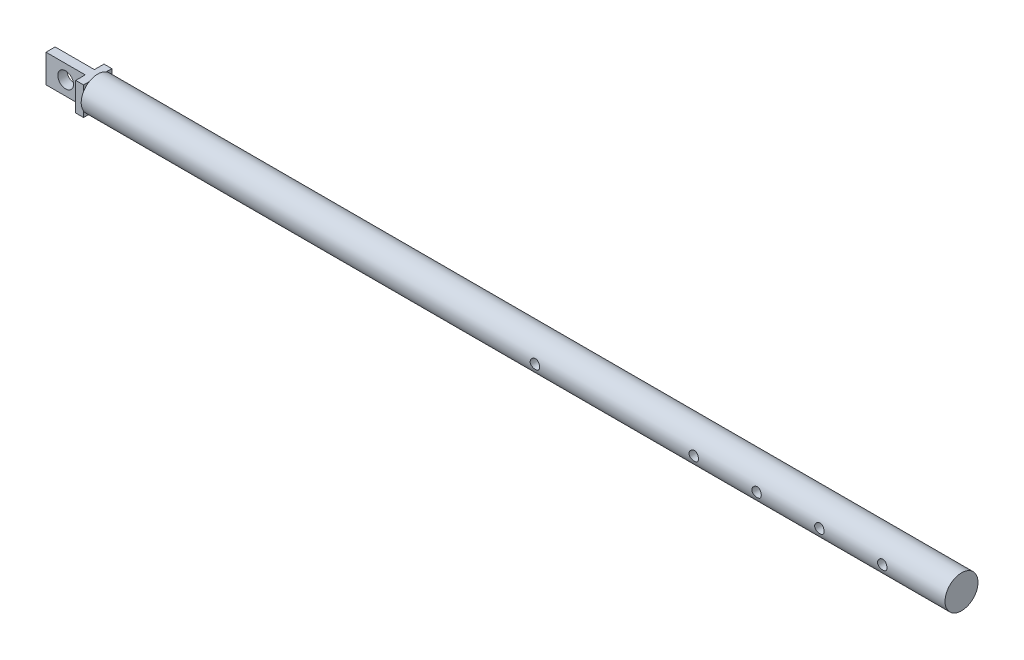
from build123d import *

# Parameters (mm, degrees)
SKETCH_1_W               = 550
SKETCH_1_H               = 10.5
CUT_EXTRUDE_1_DEPTH      = 15
CUT_EXTRUDE_1_DEPTH_BACK = 15
SKETCH_2_R               = 3
SKETCH_10_W              = 18
SKETCH_10_H              = 18
EXTRUDE_3_DEPTH          = 5
SKETCH_11_W              = 5.828442308
SKETCH_11_H              = 18
EXTRUDE_4_DEPTH          = 25
SKETCH_12_R              = 5
CUT_EXTRUDE_2_DEPTH      = 25


with BuildPart() as part:
    # 草图1 → 旋转1 (revolve)
    with BuildSketch(Plane.XY):
        with Locations((-275, 5.25)):
            Rectangle(SKETCH_1_W, SKETCH_1_H)
    revolve(axis=Axis((94.334642974, 0, 0), (-1, 0, 0)))

    # 草图2 → 切除-拉伸1 (cut, two sides: drawn at the far end of the back side and taken through both)
    with BuildSketch(Plane.XY.offset(-CUT_EXTRUDE_1_DEPTH_BACK)):
        with Locations(Location((-40, 0, 0), (0, 0, 180))):
            Circle(SKETCH_2_R)
        with Locations(Location((-80, 0, 0), (0, 0, 180))):
            Circle(SKETCH_2_R)
        with Locations(Location((-120, 0, 0), (0, 0, 180))):
            Circle(SKETCH_2_R)
        with Locations(Location((-160, 0, 0), (0, 0, 180))):
            Circle(SKETCH_2_R)
        with Locations(Location((-261.159789745, 0, 0), (0, 0, 180))):
            Circle(SKETCH_2_R)
    extrude(amount=CUT_EXTRUDE_1_DEPTH + CUT_EXTRUDE_1_DEPTH_BACK, mode=Mode.SUBTRACT)

    # 草图10 → 凸台-拉伸3 (add)
    with BuildSketch(Plane.ZY.offset(550)):
        Rectangle(SKETCH_10_W, SKETCH_10_H)
    extrude(amount=EXTRUDE_3_DEPTH)

    # 草图11 → 凸台-拉伸4 (add)
    with BuildSketch(Plane.ZY.offset(555)):
        Rectangle(SKETCH_11_W, SKETCH_11_H)
    extrude(amount=EXTRUDE_4_DEPTH)

    # 草图12 → 切除-拉伸2 (cut)
    with BuildSketch(Plane.XY.offset(2.914221154)):
        with Locations((-567.5, 0)):
            Circle(SKETCH_12_R)
    extrude(amount=-CUT_EXTRUDE_2_DEPTH, mode=Mode.SUBTRACT)


solid = part.part
